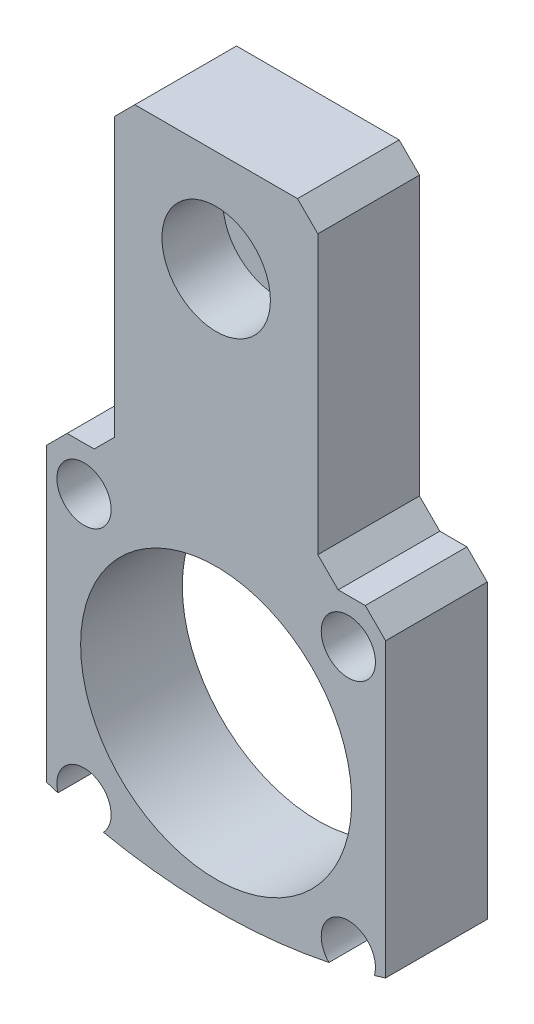
SolidWorks part; units mm, degrees
ref_plane "Front Plane" through (0, 0, 0) normal (0, 0, 1) x (1, 0, 0)
ref_plane "Top Plane" through (0, 0, 0) normal (0, 1, 0) x (1, 0, 0)
ref_plane "Right Plane" through (0, 0, 0) normal (1, 0, 0) x (0, 0, -1)
sketch "Sketch1" plane through (0, 0, 0) normal (0, 0, 1) x (1, 0, 0)
  line L1 (-25.2255, 49.6855) -> (24.7745, 49.6855)
  line L2 (-25.2255, 49.6855) -> (-25.2255, -47.3145)
  line L3 (-25.2255, -47.3145) -> (24.7745, -47.3145)
  line L4 (24.7745, 49.6855) -> (24.7745, -47.3145)
  dimension "D1" = 50
  dimension "D2" = 97
extrude "Boss-Extrude1" add sketch "Sketch1" along normal blind 15
sketch "Sketch6" plane through (0, 0, 15) normal (0, 0, 1) x (1, 0, 0)
  line L0 (-0.2255, 49.6855) -> (-0.2255, 14.7834) construction
  line L1 (24.7745, 49.6855) -> (-25.2255, 49.6855) construction
  line L2 (-25.2255, -47.3145) -> (24.7745, -47.3145) construction
  circle A0 centre (-0.2255, 34.6855) radius 8
  dimension "D2" = 16
  dimension "D1" = 82
extrude "Cut-Extrude3" cut sketch "Sketch6" against normal blind 9
sketch "Sketch7" plane through (0, 0, 6) normal (0, 0, 1) x (1, 0, 0)
  circle A0 centre (-0.2255, 34.6855) radius 4.5
  dimension "D1" = 9
extrude "Cut-Extrude4" cut sketch "Sketch7" against normal through all
sketch "Sketch8" plane through (0, 0, 0) normal (0, 0, -1) x (-1, 0, 0)
  line L0 (0.2255, -47.3145) -> (0.2255, 11.1797) construction
  line L2 (0.2255, -47.3145) -> (0.2255, 11.999) construction
  line L3 (25.2255, -47.3145) -> (-24.7745, -47.3145) construction
  line L4 (0.2255, -23.3145) -> (-37.4969, -23.3145) construction
  circle A0 centre (0.2255, -23.3145) radius 20
  circle A1 centre (-19.2745, -42.8145) radius 4
  circle A2 centre (-19.2745, -3.8145) radius 4
  circle A3 centre (19.7255, -3.8145) radius 4
  circle A4 centre (19.7255, -42.8145) radius 4
  dimension "D1" = 40
  dimension "D2" = 8
  dimension "D3" = 8
  dimension "D4" = 19.5
  dimension "D5" = 19.5
  dimension "D6" = 24
  dimension "D8" = 8
  dimension "D9" = 8
  dimension "D7" = 39
  dimension "D10" = 39
  dimension "D11" = 39
  dimension "D12" = 39
extrude "Cut-Extrude5" cut sketch "Sketch8" against normal through all
sketch "Sketch9" plane through (0, 0, 15) normal (0, 0, 1) x (1, 0, 0)
  line L0 (-25.2255, -47.3145) -> (24.7745, -47.3145) construction
  line L1 (14.7745, 64.7217) -> (46.7841, 64.7217)
  line L2 (14.7745, 64.7217) -> (14.7745, 2.6855)
  line L3 (14.7745, 2.6855) -> (46.7841, 2.6855)
  line L4 (46.7841, 64.7217) -> (46.7841, 2.6855)
  line L5 (-15.2255, 55.2568) -> (-45.6836, 55.2568)
  line L6 (-15.2255, 55.2568) -> (-15.2255, 2.6855)
  line L7 (-15.2255, 2.6855) -> (-45.6836, 2.6855)
  line L8 (-45.6836, 55.2568) -> (-45.6836, 2.6855)
  line L9 (-0.2255, 49.6855) -> (-0.2255, 34.6855) construction
  line L10 (24.7745, 49.6855) -> (-25.2255, 49.6855) construction
  dimension "D1" = 50
  dimension "D2" = 30
extrude "Cut-Extrude6" cut sketch "Sketch9" against normal through all
chamfer "Chamfer1" distance 3 angle 45 6 edges at (14.7745, 2.6855, 7.5) (-15.2255, 2.6855, 7.5) (-25.2255, 2.6855, 7.5) (24.7745, 2.6855, 7.5) (14.7745, 49.6855, 7.5) (-15.2255, 49.6855, 7.5)
sketch "Sketch14" plane through (0, 0, 0) normal (0, 0, -1) x (-1, 0, 0)
  circle A0 centre (0.2255, 34.6855) radius 82
  circle A1 centre (0.2255, 34.6855) radius 119.7203
extrude "Cut-Extrude10" cut sketch "Sketch14" against normal through all
